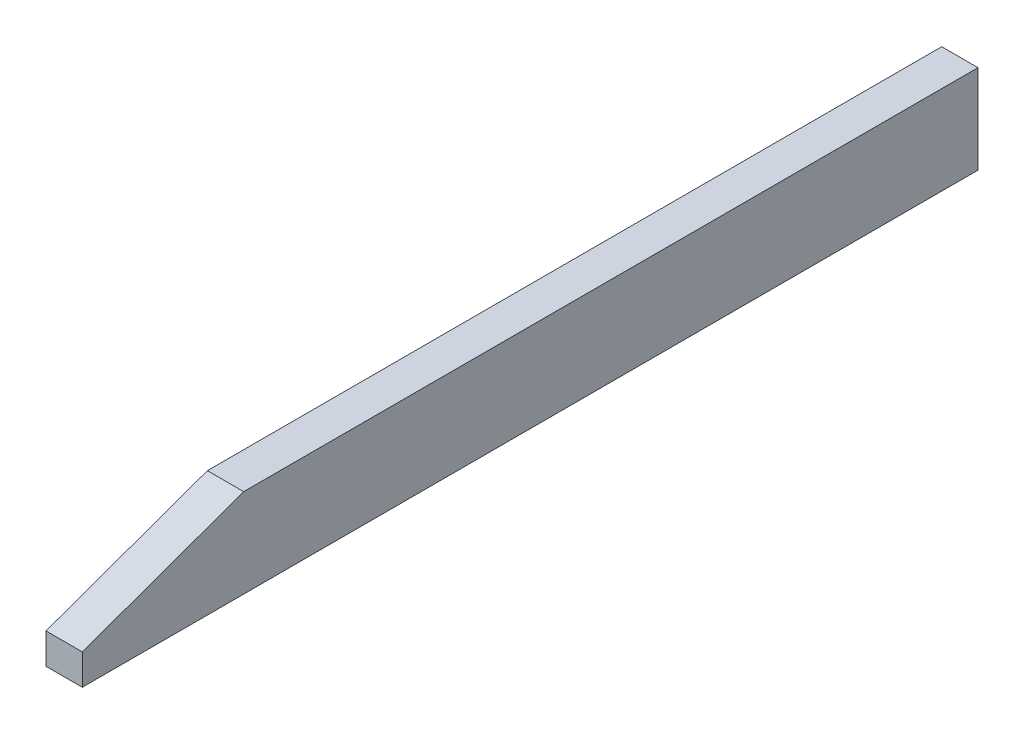
SolidWorks part; units mm, degrees
material "Q235-A"
ref_plane "Front Plane" through (0, 0, 0) normal (0, 0, 1) x (1, 0, 0)
ref_plane "Top Plane" through (0, 0, 0) normal (0, 1, 0) x (1, 0, 0)
ref_plane "Right Plane" through (0, 0, 0) normal (1, 0, 0) x (0, 0, -1)
sketch "Sketch1" plane through (0, 0, 0) normal (1, 0, 0) x (0, 0, -1)
  line L0 (0, 0) -> (1110, 0)
  line L1 (1110, 0) -> (1110, 110)
  line L2 (1110, 110) -> (200, 110)
  line L3 (200, 110) -> (0, 38)
  line L4 (0, 38) -> (0, 0)
  dimension "D1" = 1110
  dimension "D2" = 110
  dimension "D3" = 200
  dimension "D4" = 38
extrude "Boss-Extrude1" add sketch "Sketch1" along normal mid plane 45
